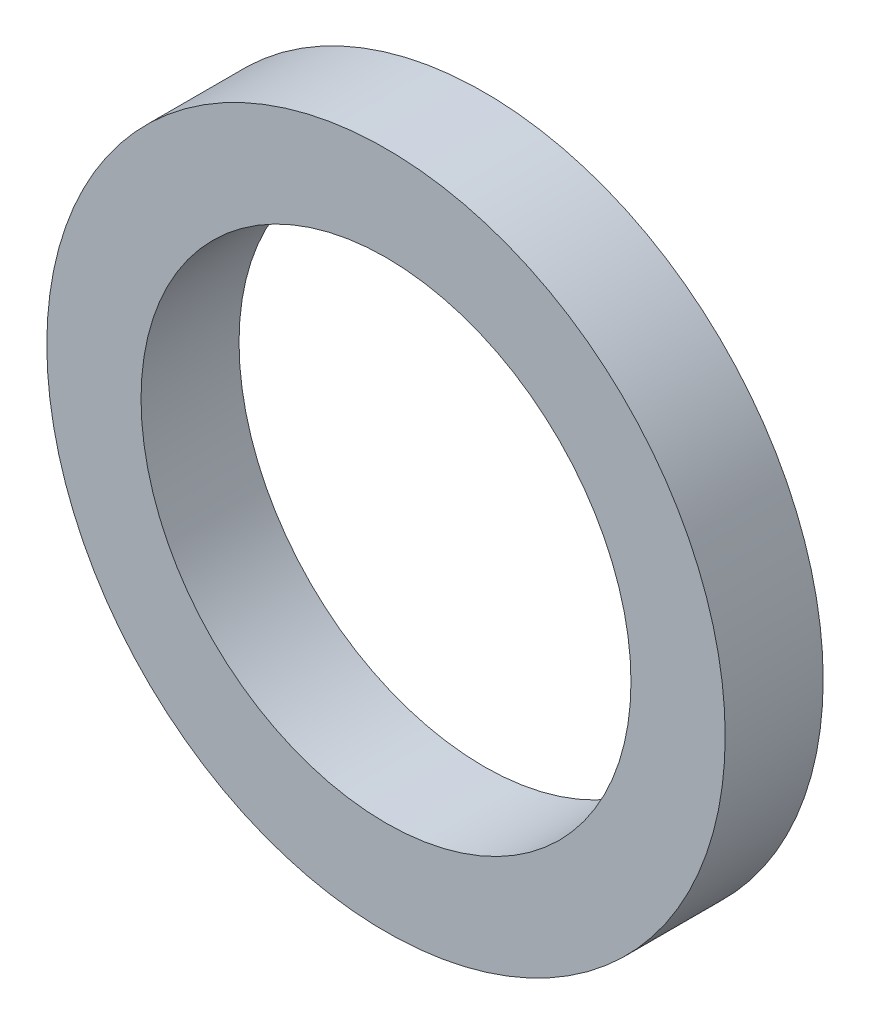
from build123d import *

# Parameters (mm, degrees)
SKETCH1_R           = 90
SKETCH1_R_2         = 65
BOSS_EXTRUDE1_DEPTH = 26


with BuildPart() as part:
    # Sketch1 → Boss-Extrude1 (new body)
    with BuildSketch(Plane.XY):
        with Locations(Location((0, 0, 0), (0, 0, 180))):
            Circle(SKETCH1_R)
        with Locations(Location((0, 0, 0), (0, 0, 180))):
            Circle(SKETCH1_R_2, mode=Mode.SUBTRACT)
    extrude(amount=BOSS_EXTRUDE1_DEPTH)


solid = part.part
